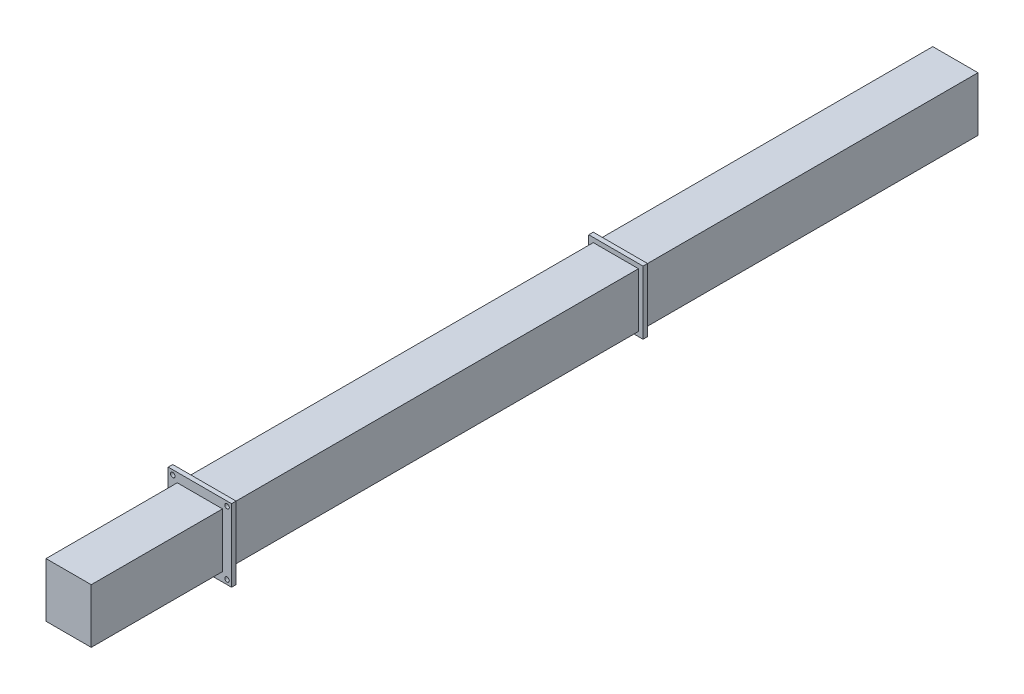
SolidWorks part; units mm, degrees
ref_plane "Front Plane" through (0, 0, 0) normal (0, 0, 1) x (1, 0, 0)
ref_plane "Top Plane" through (0, 0, 0) normal (0, 1, 0) x (1, 0, 0)
ref_plane "Right Plane" through (0, 0, 0) normal (1, 0, 0) x (0, 0, -1)
sketch "Sketch1" plane through (0, 0, 0) normal (0, 0, 1) x (1, 0, 0)
  line L0 (0, 0) -> (0, 160) construction
  line L2 (-60, 220) -> (60, 220)
  line L3 (-60, 220) -> (-60, 100)
  line L4 (-60, 100) -> (60, 100)
  line L5 (60, 220) -> (60, 100)
  line L6 (-60, 220) -> (60, 100) construction
  line L7 (-60, 100) -> (60, 220) construction
  dimension "D1" = 120
  dimension "D2" = 120
extrude "Boss-Extrude1" add sketch "Sketch1" along normal blind 700 and the other way blind 1259
sketch "Sketch2" plane through (0, 0, 700) normal (0, 0, 1) x (1, 0, 0)
  line L0 (-39.9115, 220) -> (-39.9115, 100)
  line L1 (60, 220) -> (-60, 220) construction
  line L2 (-60, 100) -> (60, 100) construction
  line L3 (-39.9115, 100) -> (-39.9115, -100) construction
  line L4 (-39.9115, 220) -> (-60, 220)
  line L5 (-60, 220) -> (-60, 100)
  line L6 (-60, 100) -> (-39.9115, 100)
extrude "Cut-Extrude1" cut sketch "Sketch2" against normal blind 2985
sketch "Sketch3" plane through (0, 0, -1259) normal (0, 0, -1) x (-1, 0, 0)
  line L0 (49.9115, 90) -> (49.9115, 230)
  line L1 (39.9115, 100) -> (-60, 100)
  line L2 (39.9115, 100) -> (39.9115, 220)
  line L3 (39.9115, 220) -> (-60, 220)
  line L4 (-60, 100) -> (-60, 220)
  line L5 (49.9115, 230) -> (-70, 230)
  line L6 (-70, 90) -> (-70, 230)
  line L7 (49.9115, 90) -> (-70, 90)
  dimension "D1" = 10
extrude "Boss-Extrude2" add sketch "Sketch3" along normal blind 10 from offset 750 offset against normal yes
sketch "Sketch4" plane through (0, 0, 700) normal (0, 0, 1) x (1, 0, 0)
  line L8 (-59.9115, 240) -> (-59.9115, 80)
  line L9 (-59.9115, 80) -> (80, 80)
  line L10 (80, 80) -> (80, 240)
  line L11 (80, 240) -> (-59.9115, 240)
  line L12 (-59.9115, 240) -> (-59.9115, 80)
  line L13 (-59.9115, 80) -> (80, 80)
  line L14 (80, 80) -> (80, 240)
  line L15 (80, 240) -> (-59.9115, 240)
  dimension "D1" = 20
extrude "Boss-Extrude3" add sketch "Sketch4" along normal blind 10 from offset 300 offset against normal yes
sketch "Sketch5" plane through (0, 0, 410) normal (0, 0, 1) x (1, 0, 0)
  line L8 (70, 230) -> (-49.9115, 230)
  line L9 (-49.9115, 230) -> (-49.9115, 90)
  line L10 (-49.9115, 90) -> (70, 90)
  line L11 (70, 90) -> (70, 230)
  line L12 (70, 230) -> (-49.9115, 230) construction
  line L13 (-49.9115, 230) -> (-49.9115, 90) construction
  line L14 (-49.9115, 90) -> (70, 90) construction
  line L15 (70, 90) -> (70, 230) construction
  circle A0 centre (70, 230) radius 5
  circle A1 centre (70, 90) radius 5
  circle A2 centre (-49.9115, 90) radius 5
  circle A3 centre (-49.9115, 230) radius 5
  dimension "D2" = 10
  dimension "D1" = 10
extrude "Cut-Extrude2" cut sketch "Sketch5" against normal blind 10
